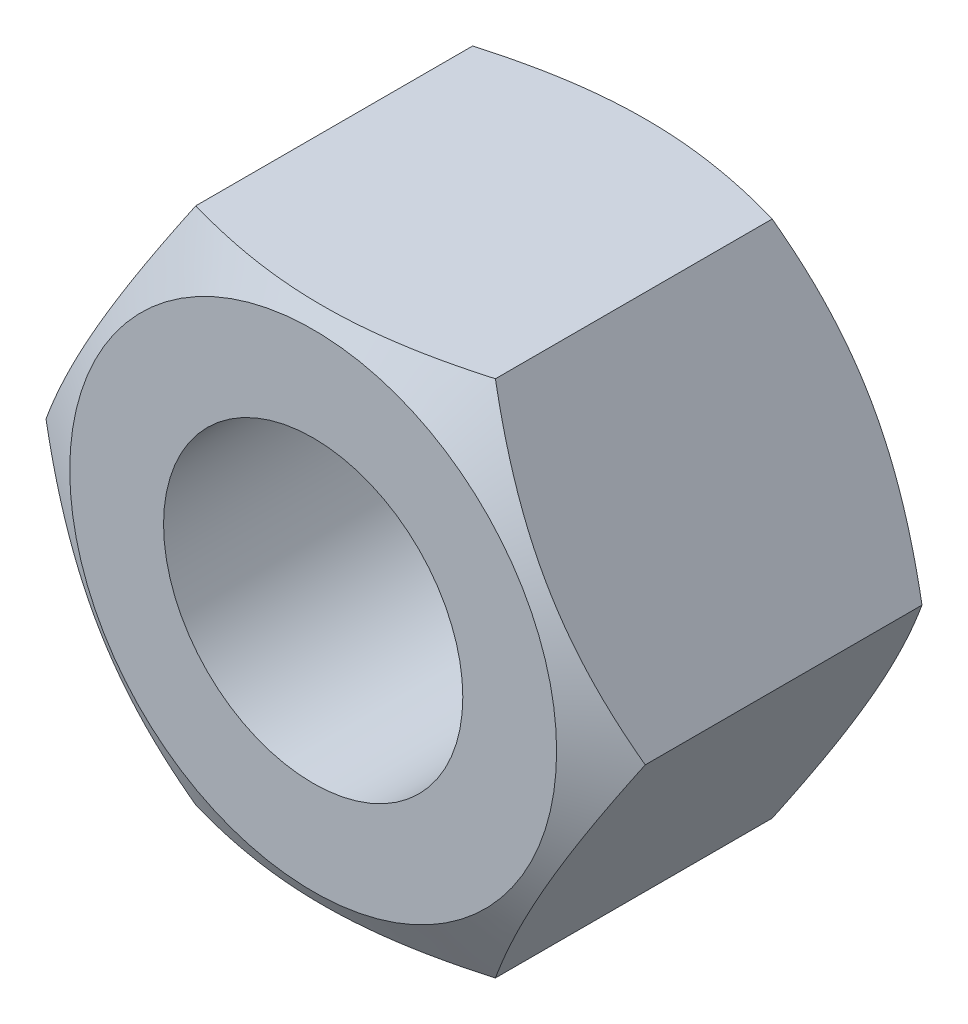
SolidWorks part; units mm, degrees
ref_plane "Front Plane" through (0, 0, 0) normal (0, 0, 1) x (1, 0, 0)
ref_plane "Top Plane" through (0, 0, 0) normal (0, 1, 0) x (1, 0, 0)
ref_plane "Right Plane" through (0, 0, 0) normal (1, 0, 0) x (0, 0, -1)
other "Configuration Table"
sketch "Sketch1" plane through (0, 0, 0) normal (0, 0, 1) x (1, 0, 0)
  line L1 (13.8564, 0) -> (6.9282, 12)
  line L2 (6.9282, 12) -> (-6.9282, 12)
  line L3 (-6.9282, 12) -> (-13.8564, 0)
  line L4 (-13.8564, 0) -> (-6.9282, -12)
  line L5 (-6.9282, -12) -> (6.9282, -12)
  line L6 (6.9282, -12) -> (13.8564, 0)
  circle A0 centre (0, 0) radius 12 construction
  dimension "D1" = 24
extrude "Boss-Extrude1" add sketch "Sketch1" along normal blind 15.8
sketch "Sketch2" plane through (0, 0, 0) normal (0, 1, 0) x (1, 0, 0)
  line L0 (-13.8564, -7.9) -> (13.8564, -7.9) construction
  line L1 (-13.8564, -15.8) -> (-13.8564, 0) construction
  line L2 (13.8564, -15.8) -> (13.8564, 0) construction
  line L3 (0, 0) -> (0, -15.8) construction
  line L4 (6.9282, -15.8) -> (-6.9282, -15.8) construction
  line L5 (13.8564, 0) -> (13.8564, -1.5) construction
  line L6 (13.8564, -1.5) -> (6.9282, 2.5)
  line L7 (13.8564, -1.5) -> (16.8564, 3.6962)
  line L8 (6.9282, 2.5) -> (16.8564, 3.6962)
  line L9 (13.8564, -14.3) -> (6.9282, -18.3)
  line L10 (13.8564, -14.3) -> (16.8564, -19.4962)
  line L11 (6.9282, -18.3) -> (16.8564, -19.4962)
revolve "Cut-Revolve1" cut sketch "Sketch2" angle 360 about L3
sketch "Sketch3" plane through (0, 0, 0) normal (0, 0, 1) x (1, 0, 0)
  circle A0 centre (0, 0) radius 6.92
extrude "Cut-Extrude1" cut sketch "Sketch3" along normal through all
cosmetic thread "Cosmetic Thread1" parameters "D2"=16
